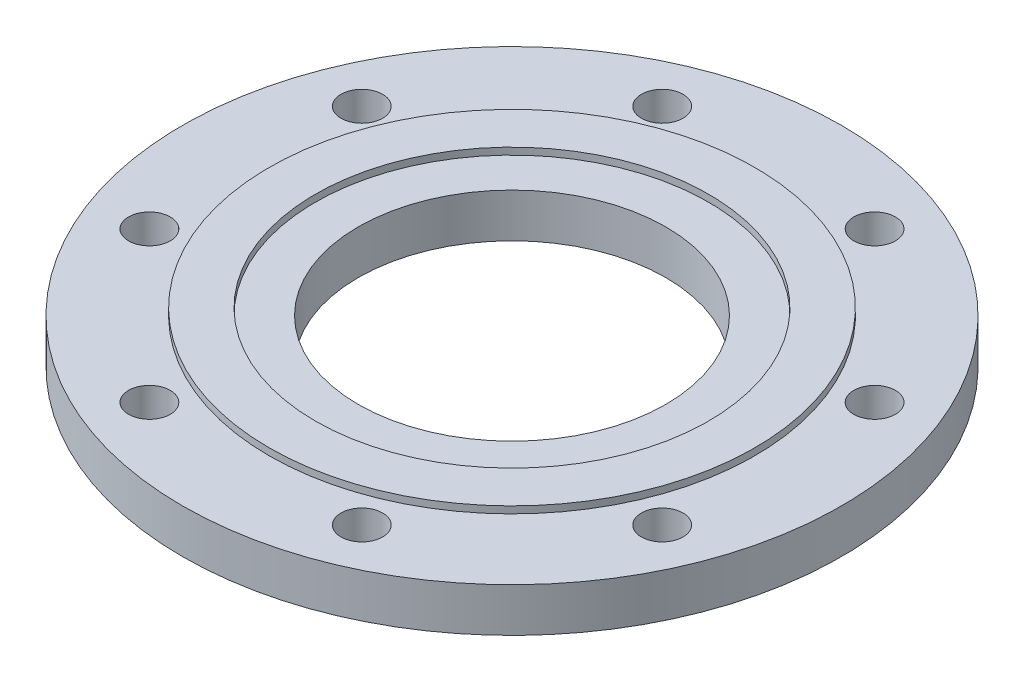
from build123d import *

# Parameters (mm, degrees)
SKETCH1_R           = 142.5
SKETCH1_R_2         = 66.5
BOSS_EXTRUDE1_DEPTH = 9.5
SKETCH2_R           = 105
SKETCH2_R_2         = 85
BOSS_EXTRUDE2_DEPTH = 3
SKETCH3_R           = 9
CUT_EXTRUDE1_DEPTH  = 203.41911965
CIRPATTERN1_COUNT   = 8


with BuildPart() as part:
    # Sketch1 → Boss-Extrude1 (new, symmetric)
    with BuildSketch(Plane(origin=(0, 0, 0), x_dir=(1, 0, 0), z_dir=(0, 1, 0))):
        with Locations(Location((0, 0, 0), (0, 0, 270))):
            Circle(SKETCH1_R)
        with Locations(Location((0, 0, 0), (0, 0, 270))):
            Circle(SKETCH1_R_2, mode=Mode.SUBTRACT)
    extrude(amount=BOSS_EXTRUDE1_DEPTH, both=True)

    # Sketch2 → Boss-Extrude2 (add)
    with BuildSketch(Plane(origin=(0, 9.5, 0), x_dir=(1, 0, 0), z_dir=(0, 1, 0))):
        with Locations(Location((0, 0, 0), (0, 0, 270))):
            Circle(SKETCH2_R)
        with Locations(Location((0, 0, 0), (0, 0, 270))):
            Circle(SKETCH2_R_2, mode=Mode.SUBTRACT)
    extrude(amount=BOSS_EXTRUDE2_DEPTH)

    # Sketch3 → Cut-Extrude1 (cut, through all)
    with BuildSketch(Plane(origin=(0, 9.5, 0), x_dir=(1, 0, 0), z_dir=(0, 1, 0))):
        with Locations(Location((-45.922011884, 110.865543901, 0), (0, 0, 270))):
            Circle(SKETCH3_R)
    cut_extrude1 = extrude(amount=-CUT_EXTRUDE1_DEPTH, mode=Mode.SUBTRACT)

    # CirPattern1: Cut-Extrude1 ×8 about axis
    cirpattern1_axis = Axis((0, 0, 0), (0, 1, 0))
    for i in range(1, CIRPATTERN1_COUNT):
        add(cut_extrude1.rotate(cirpattern1_axis, i * 360 / CIRPATTERN1_COUNT), mode=Mode.SUBTRACT)


solid = part.part
